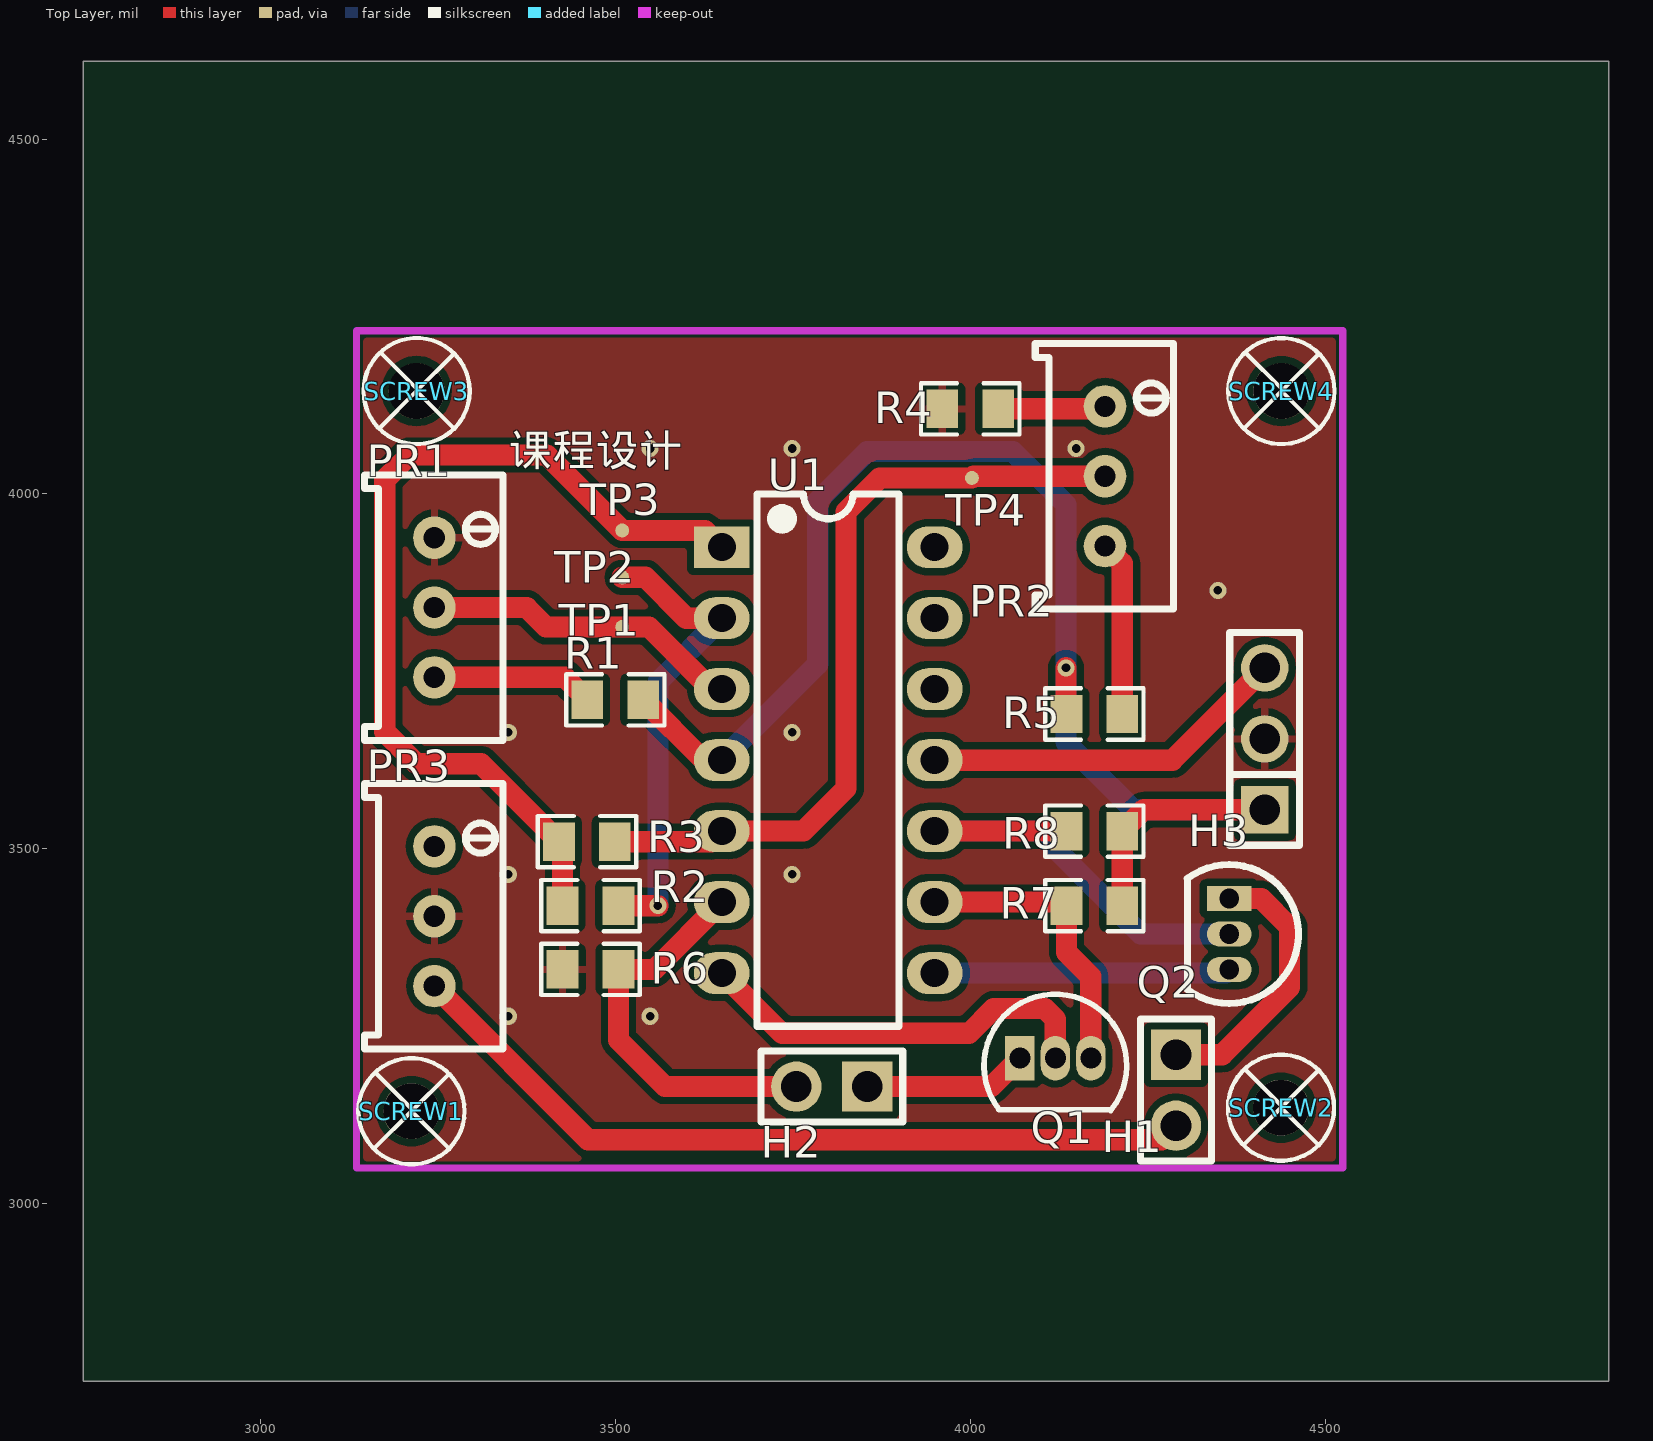
[diagram p0: Top Layer view]
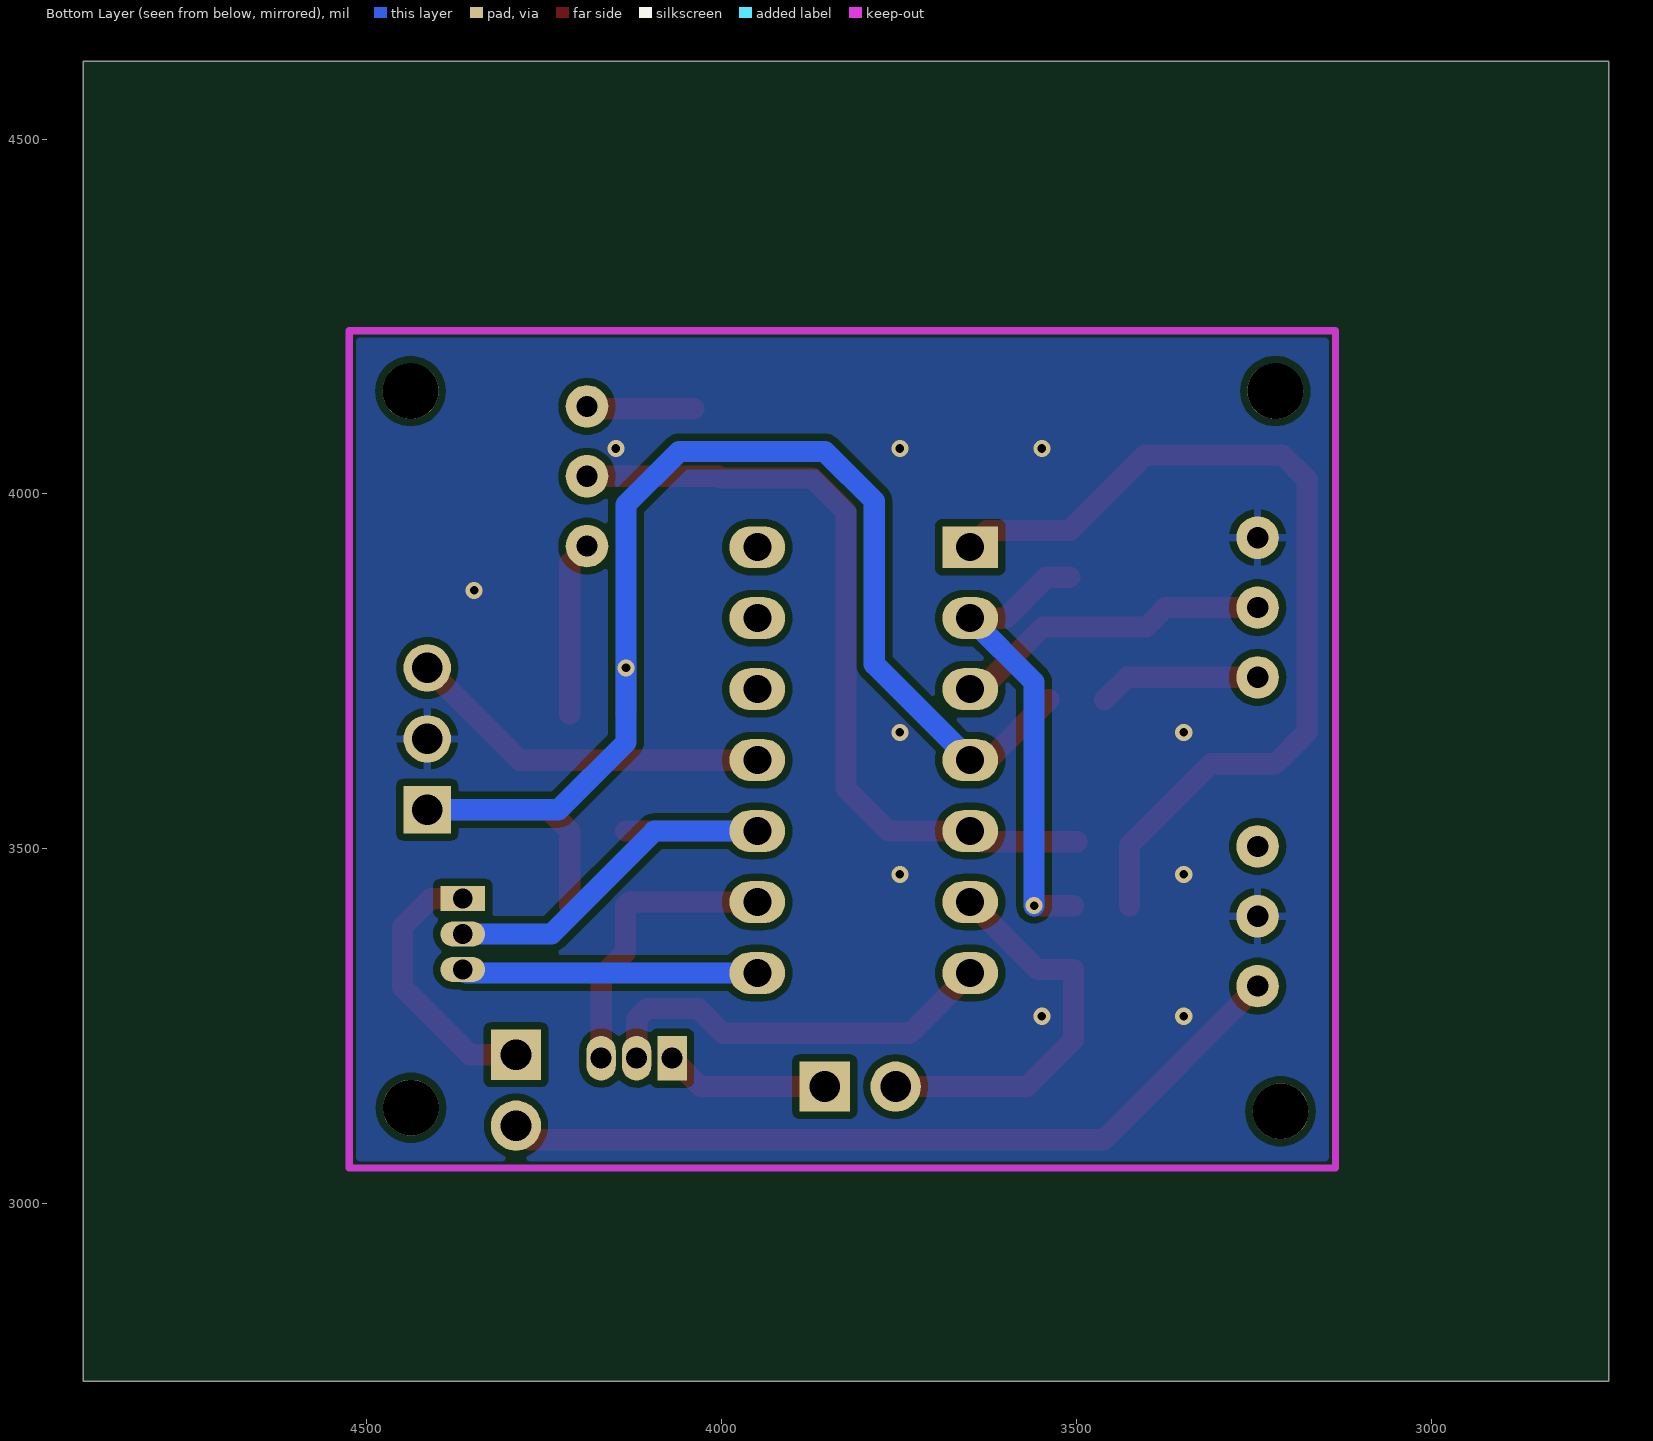
[diagram p1: Bottom Layer view, seen from below]
# Altium PCB MISC51286.pcbdoc
Units mil, origin at the board's own origin, x right, y up, seen from the top; angles counter-clockwise.
Board outline 2150 x 1860 mil, 2 copper layers (Top Layer, Bottom Layer), stack 62.206 mil thick; 25 components, 18 nets, 60 pads, 12 vias.

## Layer stack, top to bottom
Top Solder Mask Layer: solder mask 0.394, Dk 3.3
Top Layer: signal copper 1.379
Dielectric1: surface 59.449, FR4, Dk 4.5
Bottom Layer: signal copper 1.378
Bottom Solder Mask Layer: solder mask 0.394, Dk 3.3

## Board outline
4900,2750 2750,2750 2750,4610 4900,4610

## Design rules (kind name [scope] priority, off if disabled: settings)
BoardOutlineClearance copperThickness2oz_1 [All] p2 off: genericclearance=7.99 ignorepadtopadclearanceinfootprint=FALSE except(0: Arc-SplitContinuation Track-SplitContinuation SMDPad-SplitContinuation THPad-SplitContinuation Via-SplitContinuation Fill-SplitContinuation Region-SplitContinuation Poly-SplitContinuation Text-SplitContinuation Hole-SplitContinuation; 5.98: Arc-CutoutEdge SMDPad-CutoutEdge THPad-CutoutEdge Via-CutoutEdge Fill-CutoutEdge Region-CutoutEdge Text-CutoutEdge; 6.93: Hole-OutlineEdge Hole-CutoutEdge; 10: Poly-OutlineEdge Poly-CutoutEdge; 11.81: Arc-OutlineEdge Track-OutlineEdge SMDPad-OutlineEdge THPad-OutlineEdge Via-OutlineEdge Fill-OutlineEdge Region-OutlineEdge Text-OutlineEdge Track-CutoutEdge)
BoardOutlineClearance copperThickness1oz_1 [All] p4: genericclearance=4.02 ignorepadtopadclearanceinfootprint=FALSE except(0: Arc-SplitContinuation Track-SplitContinuation SMDPad-SplitContinuation THPad-SplitContinuation Via-SplitContinuation Fill-SplitContinuation Region-SplitContinuation Poly-SplitContinuation Text-SplitContinuation Hole-SplitContinuation; 6: SMDPad-CutoutEdge THPad-CutoutEdge Via-CutoutEdge Fill-CutoutEdge Region-CutoutEdge Text-CutoutEdge; 6.93: Hole-OutlineEdge Hole-CutoutEdge; 10: Poly-OutlineEdge Poly-CutoutEdge; 11.8: Arc-OutlineEdge Track-OutlineEdge SMDPad-OutlineEdge THPad-OutlineEdge Via-OutlineEdge Fill-OutlineEdge Region-OutlineEdge Text-OutlineEdge; 11.81: Arc-CutoutEdge Track-CutoutEdge)
Clearance copperThickness2oz [All] p1 off: gap=7.99 ignorepadtopadclearanceinfootprint=FALSE except(5.98: SMDPad-Track SMDPad-SMDPad THPad-Track SMDPad-THPad THPad-THPad Track-Via SMDPad-Via THPad-Via Via-Via Fill-Track Region-Track Fill-SMDPad Region-SMDPad Fill-THPad Region-THPad Fill-Via Region-Via Fill-Fill Fill-Region Region-Region Arc-Track Arc-SMDPad Arc-THPad Arc-Via Fill-Arc Region-Arc Arc-Arc Text-Track SMDPad-Text Text-THPad Text-Via Fill-Text Region-Text Arc-Text Text-Text; 6.93: Hole-Track Hole-SMDPad Hole-THPad Hole-Via Fill-Hole Region-Hole Hole-Arc Hole-Text; 10: Poly-Track Poly-SMDPad Poly-THPad Poly-Via Poly-Fill Poly-Region Poly-Poly Poly-Arc Poly-Text Poly-Hole)
Clearance copperThickness1oz [All] p3: gap=4.02 ignorepadtopadclearanceinfootprint=FALSE except(5.98: SMDPad-Track SMDPad-SMDPad THPad-Track SMDPad-THPad THPad-THPad Track-Via SMDPad-Via THPad-Via Via-Via Fill-Track Region-Track Fill-SMDPad Region-SMDPad Fill-THPad Region-THPad Fill-Via Region-Via Fill-Fill Fill-Region Region-Region; 6: Arc-Track Arc-SMDPad Arc-THPad Arc-Via Fill-Arc Region-Arc Arc-Arc Text-Track SMDPad-Text Text-THPad Text-Via Fill-Text Region-Text Arc-Text Text-Text; 6.93: Hole-Track Hole-SMDPad Hole-THPad Hole-Via Fill-Hole Region-Hole Hole-Arc Hole-Text; 10: Poly-Track Poly-SMDPad Poly-THPad Poly-Via Poly-Fill Poly-Region Poly-Poly Poly-Arc Poly-Text Poly-Hole)
DiffPairsRouting differentialPair [All] p1: maxlimit=6 minlimit=6 mostfreqgap=6 toplayer_minwidth=5 toplayer_prefwidth=10 toplayer_maxwidth=100 toplayer_mingap=6 toplayer_prefgap=6 toplayer_maxgap=6 bottomlayer_minwidth=5 bottomlayer_prefwidth=10 bottomlayer_maxwidth=100 bottomlayer_mingap=6 bottomlayer_prefgap=6 bottomlayer_maxgap=6 maxuncoupledlength=10
HoleToHoleClearance otherClearance [All] p1: gap=11.81 allowstackedmicrovias=TRUE
Length netLength [All] p1: minlimit=0 maxlimit=0
MatchedLengths netLengthTolerance [All] p1: tolerance=1000
PasteMaskExpansion pasteMaskExpansion [All] p1: expansion=0
PlaneConnect innerPlane [All] p1: planeconnectstyle=Relief reliefexpansion=20 reliefentries=4 reliefconductorwidth=10 reliefairgap=10
PolygonConnect copperRegion [(InNet('GND'))] p1: connectstyle=Relief reliefconductorwidth=10 reliefentries=4 polygonreliefangle="90 Angle" airgapwidth=10 via.connectstyle=Relief via.reliefconductorwidth=10 via.reliefentries=4 via.polygonreliefangle="90 Angle" via.airgapwidth=10
RoutingVias viaSize [All] p1: holewidth=12.01 width=24.02 viastyle="Through Hole" minholewidth=11.81 minwidth=19.68 maxholewidth=248.03 maxwidth=393.7
SolderMaskExpansion solderMaskExpansion [IsVia] p1: expansion=-1000 istentingtop=TRUE
SolderMaskExpansion solderMaskExpansion [All] p2: expansion=2 istentingtop=FALSE
Width copperThickness2oz_2 [All] p1 off: maxlimit=100 minlimit=8 preferedwidth=10
Width copperThickness1oz_2 [All] p2: maxlimit=100 minlimit=5 preferedwidth=10

## Components (designator, comment, footprint, x,y, rotation, side; value= is the part's Value field where it differs from the comment)
H1 "" HDR-TH_2P-P2.54-V-M-1 4290,3160 r270 top
H2 "" HDR-TH_2P-P2.54-V-M-1 3805,3165 r180 top
H3 "" HDR-TH_3P-P2.54-V-M 4415,3655 r90 top
PR1 "20kΩ" R_3296 3250,3840 r270 top
PR2 "10kΩ" R_3296 4195,4025 r270 top
PR3 "250" R_3296 3250,3405 r270 top
Q1 "2N2222A" TO-92-3_L5.1-W4.1-P1.27-L-1 4120,3205 r0 top
Q2 "2SA1015(RANGE:200-400)" TO-92-3_L4.9-W3.7-P1.27-L 4365,3380 r270 top
R1 "40K" R0805 3500,3710 r0 top
R2 "1K" R0805 3465,3420 r0 top
R3 "1K" R0805 3460,3510 r180 top
R4 "1K" R0805 4000,4120 r180 top
R5 "10K" R0805 4175,3690 r0 top
R6 "249" R0805 3465,3330 r180 top
R7 "804" R0805 4175,3420 r180 top
R8 "804" R0805 4175,3525 r180 top
SCREW1 "" M2螺丝 3212.7,3130.25 r0 top
SCREW2 "" M2螺丝 4437.98,3135.25 r0 top
SCREW3 "" M2螺丝 3220,4145 r0 top
SCREW4 "" M2螺丝 4438.56,4144.96 r0 top
TP1 "" Test-Point-0.5mm 3509.69,3812.58 r180 top
TP2 "" Test-Point-0.5mm 3509.69,3882.58 r90 top
TP3 "" Test-Point-0.5mm 3509.69,3948.68 r90 top
TP4 "" Test-Point-0.5mm 4002.32,4022.58 r0 top
U1 "LM324N196" PDIP-14_L19.3-W6.5-P2.54-LS7.6-BL 3800,3625 r270 top

## Footprints (in the part's own frame and the unit in brackets; to place one, negate y for a bottom-side part, rotate by r counter-clockwise, add the part's x,y. Pads: shape width x height; smd on the part's side, far side on the other; paste and mask are expansions set on the pad)
HDR-TH_2P-P2.54-V-M-1 [mm]
  rect 1.8x1.8 hole 1.1: 1(-1.27,0)
  round 1.8 hole 1.1: 2(1.27,0)
  silkscreen extent -2.54,-1.27 2.54,1.27
HDR-TH_3P-P2.54-V-M [mm]
  rect 1.7x1.7 hole 1.1: 1(-2.54,0)
  round 1.7 hole 1.1: 2(0,0) 3(2.54,0)
  silkscreen extent -3.81,-1.25 3.81,1.25
M2螺丝 [mm]
  round 2 hole 2: 1(0,0)
  silkscreen extent -1.9,-1.9 1.9,1.9
PDIP-14_L19.3-W6.5-P2.54-LS7.6-BL [mm]
  rect 1.5x2 hole 1: 1(-7.62,-3.81)
  oval 1.5x2 hole 1: 2(-5.08,-3.81) 3(-2.54,-3.81) 4(0,-3.81) 5(2.54,-3.81) 6(5.08,-3.81) 7(7.62,-3.81) 8(7.62,3.81) 9(5.08,3.81) 10(2.54,3.81) 11(0,3.81) 12(-2.54,3.81) 13(-5.08,3.81) 14(-7.62,3.81)
  silkscreen extent -9.53,-2.55 9.53,2.53
R0805 [mm]
  rect 1.133x1.377 smd paste-100 mask+0.051: 1(-1,0) 2(1,0)
  silkscreen extent -1.76,-0.92 1.76,0.92
R_3296 [mil]
  round 60 hole 30 paste+0 mask+2: 1(-98.4,-5) 2(0,-5) 3(98.4,-5)
  silkscreen extent -187,-103 187,92
Test-Point-0.5mm [mm]
  round 0.5 smd: 1(0,0)
TO-92-3_L4.9-W3.7-P1.27-L [mm]
  rect 0.9x1.6 hole 0.7: 1(-1.27,0)
  oval 0.9x1.6 hole 0.7: 2(0,0) 3(1.27,0)
  silkscreen extent -2.48,-1.5 2.48,2.48
TO-92-3_L5.1-W4.1-P1.27-L-1 [mm]
  rect 1.05x1.6 hole 0.75: 1(-1.27,0)
  oval 1.05x1.6 hole 0.75: 2(0,0) 3(1.27,0)
  silkscreen extent -2.55,-1.87 2.55,2.29

## Via types
v1: diameter 24.02, hole 12, Top Layer to Bottom Layer, 12 vias

## Nets (pads, with @x,y where several pads share a name; then routed paths per layer and width w, separated by ;. In a path a pad name is that pad's centre, name@x,y a point inside that pad or via, vN(x,y) a via of type N, cw(c..) or ccw(c..) an arc to the next point about the centre after c; other vN are vias at no path point)
15V: H3.1 R1.2 R5.1 R7.1 R8.1 U1.4 | length 2014.5
  Top Layer w30: R1.2 3624.37,3625 U1.4 ; v1(4135,3755) 4135,3690.63 R5.1 ; R7.1 R8.1 4244.37,3555 H3.1
  Bottom Layer w30: U1.4 3785,3760 3785,3990 3855,4060 4060,4060 4135,3985 v1(4135,3755) 4135,3650 4230,3555 H3.1
$1N2: PR1.3 R1.1 | length 228.7
  Top Layer w30: PR1.3 3429.03,3741.6 R1.1
$1N4: PR1.2 TP1.1 U1.3 | length 452.6
  Top Layer w30: PR1.2 3375,3840 3402.42,3812.58 TP1.1 3547.42,3812.58 3635,3725 U1.3
$1N8: R2.2 TP2.1 U1.2 | length 662.1
  Top Layer w30: R2.2 v1(3560,3420) ; TP2.1 3542.42,3882.58 3600,3825 U1.2
  Bottom Layer w30: v1(3560,3420) 3560,3735 U1.2
$1N9: R2.1 R3.2 TP3.1 U1.1 | length 1300.2
  Top Layer w30: R2.1 3425.63,3505 R3.2 3310.63,3620 3220,3620 3175,3665 3175,4020 3210,4055 3403.37,4055 TP3.1 3626.32,3948.68 U1.1
$1N10: PR2.2 R3.1 TP4.1 U1.5 | length 1132.3
  Top Layer w30: R3.1 3635,3510 U1.5 3765,3525 3825,3585 3825,3975 3872.58,4022.58 TP4.1 ; TP4.1@4002.39,4022.65 4004.74,4025 PR2.2
$1N11: PR2.1 R4.1 | length 152
  Top Layer w30: R4.1 4186.6,4120 PR2.1
$1N13: PR2.3 R5.2 | length 246.7
  Top Layer w30: PR2.3 4214.37,3902.23 R5.2
$1N17: Q1.2 U1.7 | length 580.9
  Top Layer w30: U1.7 3735,3240 3998.24,3240 4033.24,3275 4105,3275 4120,3260 Q1.2
$1N18: Q1.3 R7.2 U1.9 | length 416.9
  Top Layer w30: U1.9 4130.63,3425 R7.2 4135.63,3354.37 4170,3320 Q1.3
$1N20: Q2.2 R8.2 U1.10 | length 660.7
  Top Layer w30: U1.10 R8.2
  Bottom Layer w30: U1.10 4095,3525 4240,3380 Q2.2
$1N22: Q2.3 U1.8 | length 417.1
  Bottom Layer w30: U1.8 4360,3325 Q2.3
$1N23: H1.1 Q2.1 | length 385.9
  Top Layer w30: H1.1 4355,3210 4450,3305 4450,3390 4410,3430 Q2.1
$1N24: H1.2 PR3.3 | length 1143
  Top Layer w30: PR3.3 3461.6,3090 4270,3090 H1.2
$1N26: H2.1 Q1.1 | length 231.6
  Top Layer w30: H2.1 4030,3165 Q1.1
$1N27: H2.2 R6.1 U1.6 | length 562.2
  Top Layer w30: U1.6 3555,3330 R6.1 3504.37,3230.63 3570,3165 H2.2
-15V: H3.3 U1.11 | length 518.8
  Top Layer w30: U1.11 4285,3625 H3.3
GND: H3.2 PR1.1 PR3.2 R4.2 R6.2
  other v1: 3349.1,3264.1 3549.1,3264.1 3349.1,3464.1 3749.1,3464.1 3349.1,3664.1 3749.1,3664.1 4349.1,3864.1 3549.1,4064.1 3749.1,4064.1 4149.1,4064.1
pads on no net: PR3.1 SCREW1.1 SCREW2.1 SCREW3.1 SCREW4.1 U1.12 U1.13 U1.14

## Polygon pours and split planes (outlines as drawn)
GND on Top Layer (solid, remove dead copper, pour order 0): 3000,4360 3000,3000 4650,3000 4650,4360
GND on Bottom Layer (solid, remove dead copper, pour order 2): 3060,4320 3060,3010 4600,3010 4600,4320

## Keep-outs
Board Outline Layer:
  lines w10: 3135,3050 3135,4230 4525,4230 4525,3050 3135,3050

## Silkscreen, mask and mechanical layers (free items; w line width, h text height)
Top Silkscreen Layer:
  text "课程设计" at 3350,4040 h45